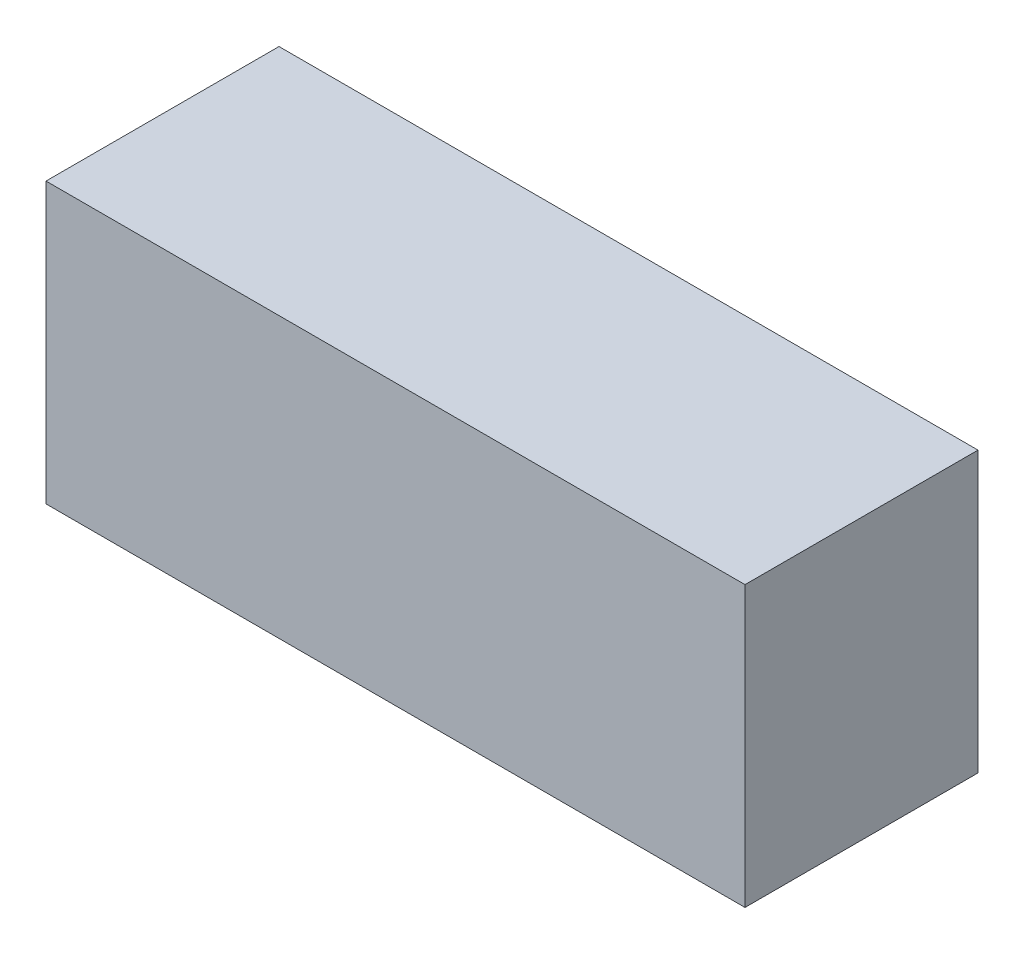
SolidWorks part; units mm, degrees
ref_plane "前视基准面" through (0, 0, 0) normal (0, 0, 1) x (1, 0, 0)
ref_plane "上视基准面" through (0, 0, 0) normal (0, 1, 0) x (1, 0, 0)
ref_plane "右视基准面" through (0, 0, 0) normal (1, 0, 0) x (0, 0, -1)
other "Configuration Table"
sketch "草图1" plane through (0, 0, 0) normal (0, 0, 1) x (1, 0, 0)
  line L0 (-15, -6) -> (15, -6)
  line L1 (15, -6) -> (15, 6)
  line L2 (15, 6) -> (-15, 6)
  line L3 (-15, 6) -> (-15, -6)
  point P0 (0, 0)
  dimension "D1" = 15
  dimension "D2" = 30
  dimension "D3" = 6
  dimension "D4" = 12
extrude "凸台-拉伸1" add sketch "草图1" against normal mid plane 10
